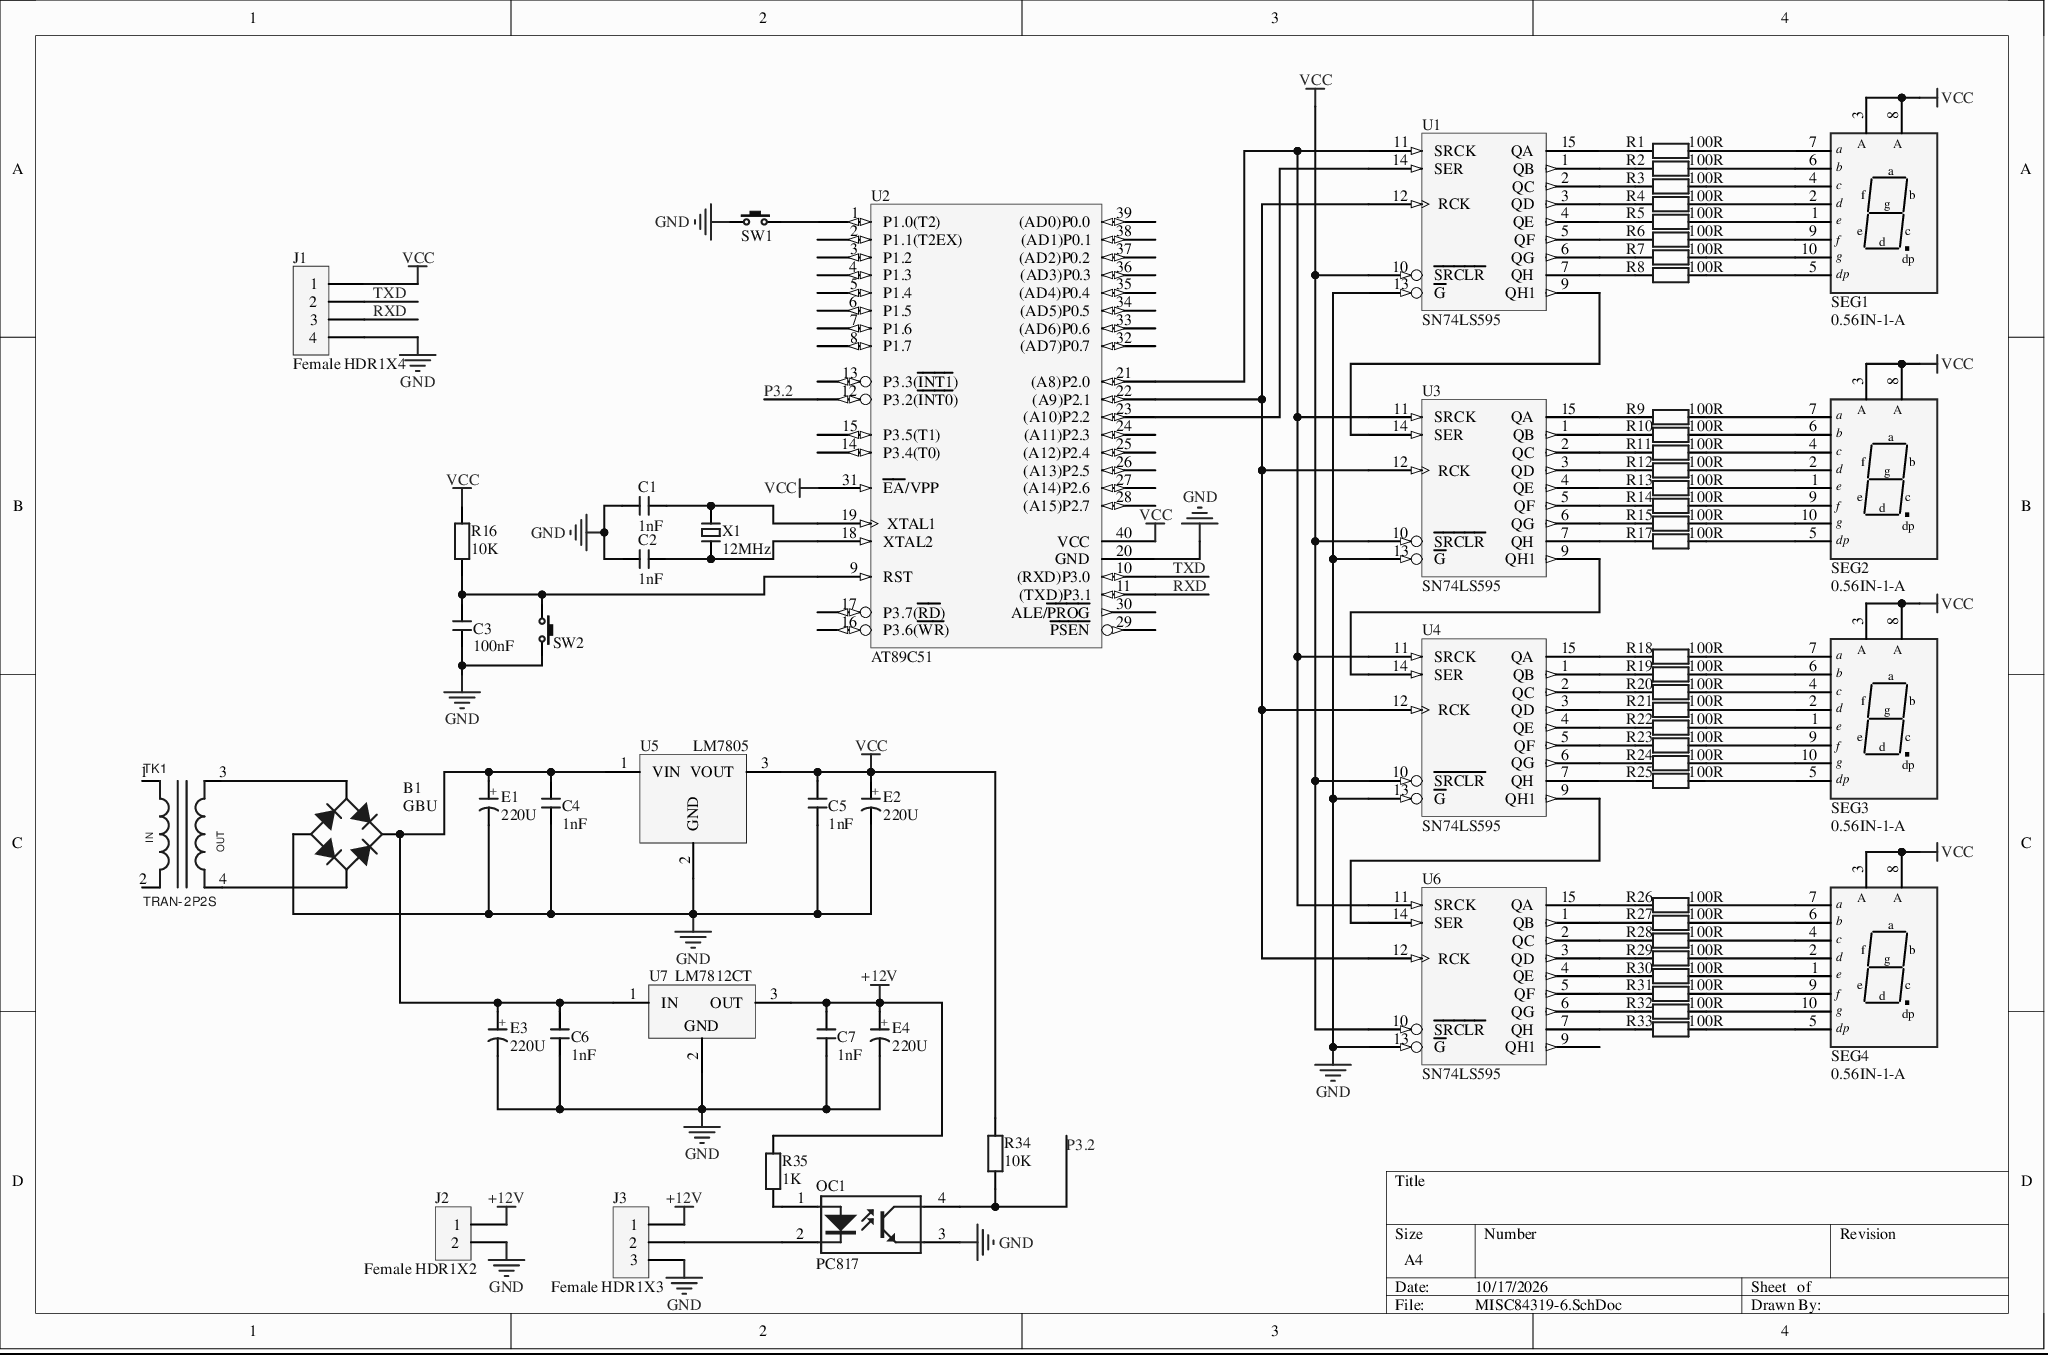
[diagram p0: MISC84319-6.SchDoc]
# Altium project MISC84319-2.PrjPcb
1 sheet, 66 parts. Net scope: global (net labels, ports and power ports of the same name join across sheets).
Board file: MISC84319.PcbDoc

## Sheet MISC84319-6.SchDoc
size A4

### Parts
B1  GBU  [GBU]
C1  1nF  [CC 1.8*3.6]
C2  1nF  [CC 1.8*3.6]
C3  100nF  [CC 1.8*3.6]
C4  1nF  [CC 1.8*3.6]
C5  1nF  [CC 1.8*3.6]
C6  1nF  [CC 1.8*3.6]
C7  1nF  [CC 1.8*3.6]
E1  220U  [CS 2.0*5*8 - C]
E2  220U  [CS 2.0*5*8 - C]
E3  220U  [CS 2.0*5*8 - C]
E4  220U  [CS 2.0*5*8 - C]
J1  Female HDR1X4  [Fe-HDR1X4/2.54-S]
J2  Female HDR1X2  [Fe-HDR1X2/2.54-S]
J3  Female HDR1X3  [Fe-HDR1X3/2.54-S]
OC1  PC817  [DIP_PC817]
R1  100R  [RS 1/4W]
R2  100R  [RS 1/4W]
R3  100R  [RS 1/4W]
R4  100R  [RS 1/4W]
R5  100R  [RS 1/4W]
R6  100R  [RS 1/4W]
R7  100R  [RS 1/4W]
R8  100R  [RS 1/4W]
R9  100R  [RS 1/4W]
R10  100R  [RS 1/4W]
R11  100R  [RS 1/4W]
R12  100R  [RS 1/4W]
R13  100R  [RS 1/4W]
R14  100R  [RS 1/4W]
R15  100R  [RS 1/4W]
R16  10K  [RS 1/4W]
R17  100R  [RS 1/4W]
R18  100R  [RS 1/4W]
R19  100R  [RS 1/4W]
R20  100R  [RS 1/4W]
R21  100R  [RS 1/4W]
R22  100R  [RS 1/4W]
R23  100R  [RS 1/4W]
R24  100R  [RS 1/4W]
R25  100R  [RS 1/4W]
R26  100R  [RS 1/4W]
R27  100R  [RS 1/4W]
R28  100R  [RS 1/4W]
R29  100R  [RS 1/4W]
R30  100R  [RS 1/4W]
R31  100R  [RS 1/4W]
R32  100R  [RS 1/4W]
R33  100R  [RS 1/4W]
R34  10K  [RS 1/4W]
R35  1K  [RS 1/4W]
SEG1  0.56IN-1-A  [0.56IN-1P]
SEG2  0.56IN-1-A  [0.56IN-1P]
SEG3  0.56IN-1-A  [0.56IN-1P]
SEG4  0.56IN-1-A  [0.56IN-1P]
SW1  3x6x5  [TSW DIP-3*6*5]  (value not drawn)
SW2  3x6x5  [TSW DIP-3*6*5]  (value not drawn)
TK1  TRAN-2P2S  [TRANS2P2S]
U1  SN74LS595  [DIP-16]
U2  AT89C51  [DIP40]
U3  SN74LS595  [DIP-16]
U4  SN74LS595  [DIP-16]
U5  LM7805  [TO220A]
U6  SN74LS595  [DIP-16]
U7  LM7812CT  [T03B]
X1  12MHz  [OSC HC-49S]

### Nets
+12V: C7.2 E4.1(A) J2.1 J3.1 R35.2 U7.3(OUT)
GND: B1.DC- C1.1 C2.1 C3.1 C4.1 C5.1 C6.1 C7.1 E1.2(K) E2.2(K) E3.2(K) E4.2(K) J1.4 J2.2 J3.3 OC1.3(E) SW1.1 SW2.2 U1.8(GND) U1.13(~{G}) U2.20(GND) U3.8(GND) U3.13(~{G}) U4.8(GND) U4.13(~{G}) U5.2(GND) U6.8(GND) U6.13(~{G}) U7.2(GND)
VCC: C5.2 E2.1(A) J1.1 R16.2 R34.2 SEG1.3(VCC) SEG1.8 SEG2.3(VCC) SEG2.8 SEG3.3(VCC) SEG3.8 SEG4.3(VCC) SEG4.8 U1.10(~{SRCLR}) U1.16(VCC) U2.31(~{EA}/VPP) U2.40(VCC) U3.10(~{SRCLR}) U3.16(VCC) U4.10(~{SRCLR}) U4.16(VCC) U5.3(VOUT) U6.10(~{SRCLR}) U6.16(VCC)
P3.2: OC1.4(C) R34.1 U2.12(P3.2(~{INT0}))
RXD: J1.3 U2.11((TXD)P3.1)
TXD: J1.2 U2.10((RXD)P3.0)
NetB1_AC1: B1.AC1 TK1.3(Sec+)
NetB1_AC2: B1.AC2 TK1.4(Sec-)
NetB1_DC+: B1.DC+ C4.2 C6.2 E1.1(A) E3.1(A) U5.1(VIN) U7.1(IN)
NetC1_2: C1.2 U2.19(XTAL1) X1.2
NetC2_2: C2.2 U2.18(XTAL2) X1.1
NetC3_2: C3.2 R16.1 SW2.1 U2.9(RST)
NetJ3_2: J3.2 OC1.2(K)
NetOC1_1: OC1.1(A) R35.1
NetR1_1: R1.1 U1.15(QA)
NetR1_2: R1.2 SEG1.7
NetR2_1: R2.1 U1.1(QB)
NetR2_2: R2.2 SEG1.6
NetR3_1: R3.1 U1.2(QC)
NetR3_2: R3.2 SEG1.4
NetR4_1: R4.1 U1.3(QD)
NetR4_2: R4.2 SEG1.2
NetR5_1: R5.1 U1.4(QE)
NetR5_2: R5.2 SEG1.1
NetR6_1: R6.1 U1.5(QF)
NetR6_2: R6.2 SEG1.9
NetR7_1: R7.1 U1.6(QG)
NetR7_2: R7.2 SEG1.10
NetR8_1: R8.1 U1.7(QH)
NetR8_2: R8.2 SEG1.5
NetR9_1: R9.1 U3.15(QA)
NetR9_2: R9.2 SEG2.7
NetR10_1: R10.1 U3.1(QB)
NetR10_2: R10.2 SEG2.6
NetR11_1: R11.1 U3.2(QC)
NetR11_2: R11.2 SEG2.4
NetR12_1: R12.1 U3.3(QD)
NetR12_2: R12.2 SEG2.2
NetR13_1: R13.1 U3.4(QE)
NetR13_2: R13.2 SEG2.1
NetR14_1: R14.1 U3.5(QF)
NetR14_2: R14.2 SEG2.9
NetR15_1: R15.1 U3.6(QG)
NetR15_2: R15.2 SEG2.10
NetR17_1: R17.1 U3.7(QH)
NetR17_2: R17.2 SEG2.5
NetR18_1: R18.1 U4.15(QA)
NetR18_2: R18.2 SEG3.7
NetR19_1: R19.1 U4.1(QB)
NetR19_2: R19.2 SEG3.6
NetR20_1: R20.1 U4.2(QC)
NetR20_2: R20.2 SEG3.4
NetR21_1: R21.1 U4.3(QD)
NetR21_2: R21.2 SEG3.2
NetR22_1: R22.1 U4.4(QE)
NetR22_2: R22.2 SEG3.1
NetR23_1: R23.1 U4.5(QF)
NetR23_2: R23.2 SEG3.9
NetR24_1: R24.1 U4.6(QG)
NetR24_2: R24.2 SEG3.10
NetR25_1: R25.1 U4.7(QH)
NetR25_2: R25.2 SEG3.5
NetR26_1: R26.1 U6.15(QA)
NetR26_2: R26.2 SEG4.7
NetR27_1: R27.1 U6.1(QB)
NetR27_2: R27.2 SEG4.6
NetR28_1: R28.1 U6.2(QC)
NetR28_2: R28.2 SEG4.4
NetR29_1: R29.1 U6.3(QD)
NetR29_2: R29.2 SEG4.2
NetR30_1: R30.1 U6.4(QE)
NetR30_2: R30.2 SEG4.1
NetR31_1: R31.1 U6.5(QF)
NetR31_2: R31.2 SEG4.9
NetR32_1: R32.1 U6.6(QG)
NetR32_2: R32.2 SEG4.10
NetR33_1: R33.1 U6.7(QH)
NetR33_2: R33.2 SEG4.5
NetSW1_2: SW1.2 U2.1(P1.0(T2))
NetU1_9: U1.9(QH1) U3.14(SER)
NetU1_11: U1.11(SRCK) U2.21((A8)P2.0) U3.11(SRCK) U4.11(SRCK) U6.11(SRCK)
NetU1_12: U1.12(RCK) U2.22((A9)P2.1) U3.12(RCK) U4.12(RCK) U6.12(RCK)
NetU1_14: U1.14(SER) U2.23((A10)P2.2)
NetU3_9: U3.9(QH1) U4.14(SER)
NetU4_9: U4.9(QH1) U6.14(SER)

Not connected (* = marked no-connect by the designer): TK1 1(Pri+) 2(Pri-); U2 2(P1.1(T2EX)) 3(P1.2) 4(P1.3) 5(P1.4) 6(P1.5) 7(P1.6) 8(P1.7) 13(P3.3(~{INT1})) 14(P3.4(T0)) 15(P3.5(T1)) 16(P3.6(~{WR})) 17(P3.7(~{RD})) 24((A11)P2.3) 25((A12)P2.4) 26((A13)P2.5) 27((A14)P2.6) 28((A15)P2.7) 29(~{PSEN}) 30(ALE/~{PROG}) 32((AD7)P0.7) 33((AD6)P0.6) 34((AD5)P0.5) 35((AD4)P0.4) 36((AD3)P0.3) 37((AD2)P0.2) 38((AD1)P0.1) 39((AD0)P0.0); U6 9(QH1)

### Library data of the parts
B1 = GBU: 1kV/10A bridge rectifier; BOM名称: 1kV/10A bridge rectifier
C1-C7 = CC: ceramic disc capacitor; BOM名称: Through-hole ceramic disc capacitor
E1-E4 = CS: through-hole solid-state capacitor; BOM名称: through-hole solid-state capacitor
OC1 = PC817: linear optocoupler
R1-R35 = R-S: colour-band resistor; BOM名称: colour-band resistor
SEG1-SEG4 = 0.56IN-1-A: 1-digit 0.56 inch common-anode display
SW1 SW2 = TSW 3x6: 3x6 tact switch; BOM名称: 3x6 tact switch
U1 U3 U4 U6 = SN74LS595: 8-BIT SFT REG WIRTH OUTPUT LCH
U2 = STC89C51
U7 = LM7812CT: Series 3-Terminal Positive Regulator; Package Information: Latest Revision: 1995; Note: Tab is connected to GND; Published: 15-Apr-2002; Datasheet: Latest Revision: May-1999; Package Reference: T03B; Publisher: Altium Limited
X1 = XTAL-2P: 2-pin passive crystal oscillator; BOM名称: 2-pin passive crystal oscillator